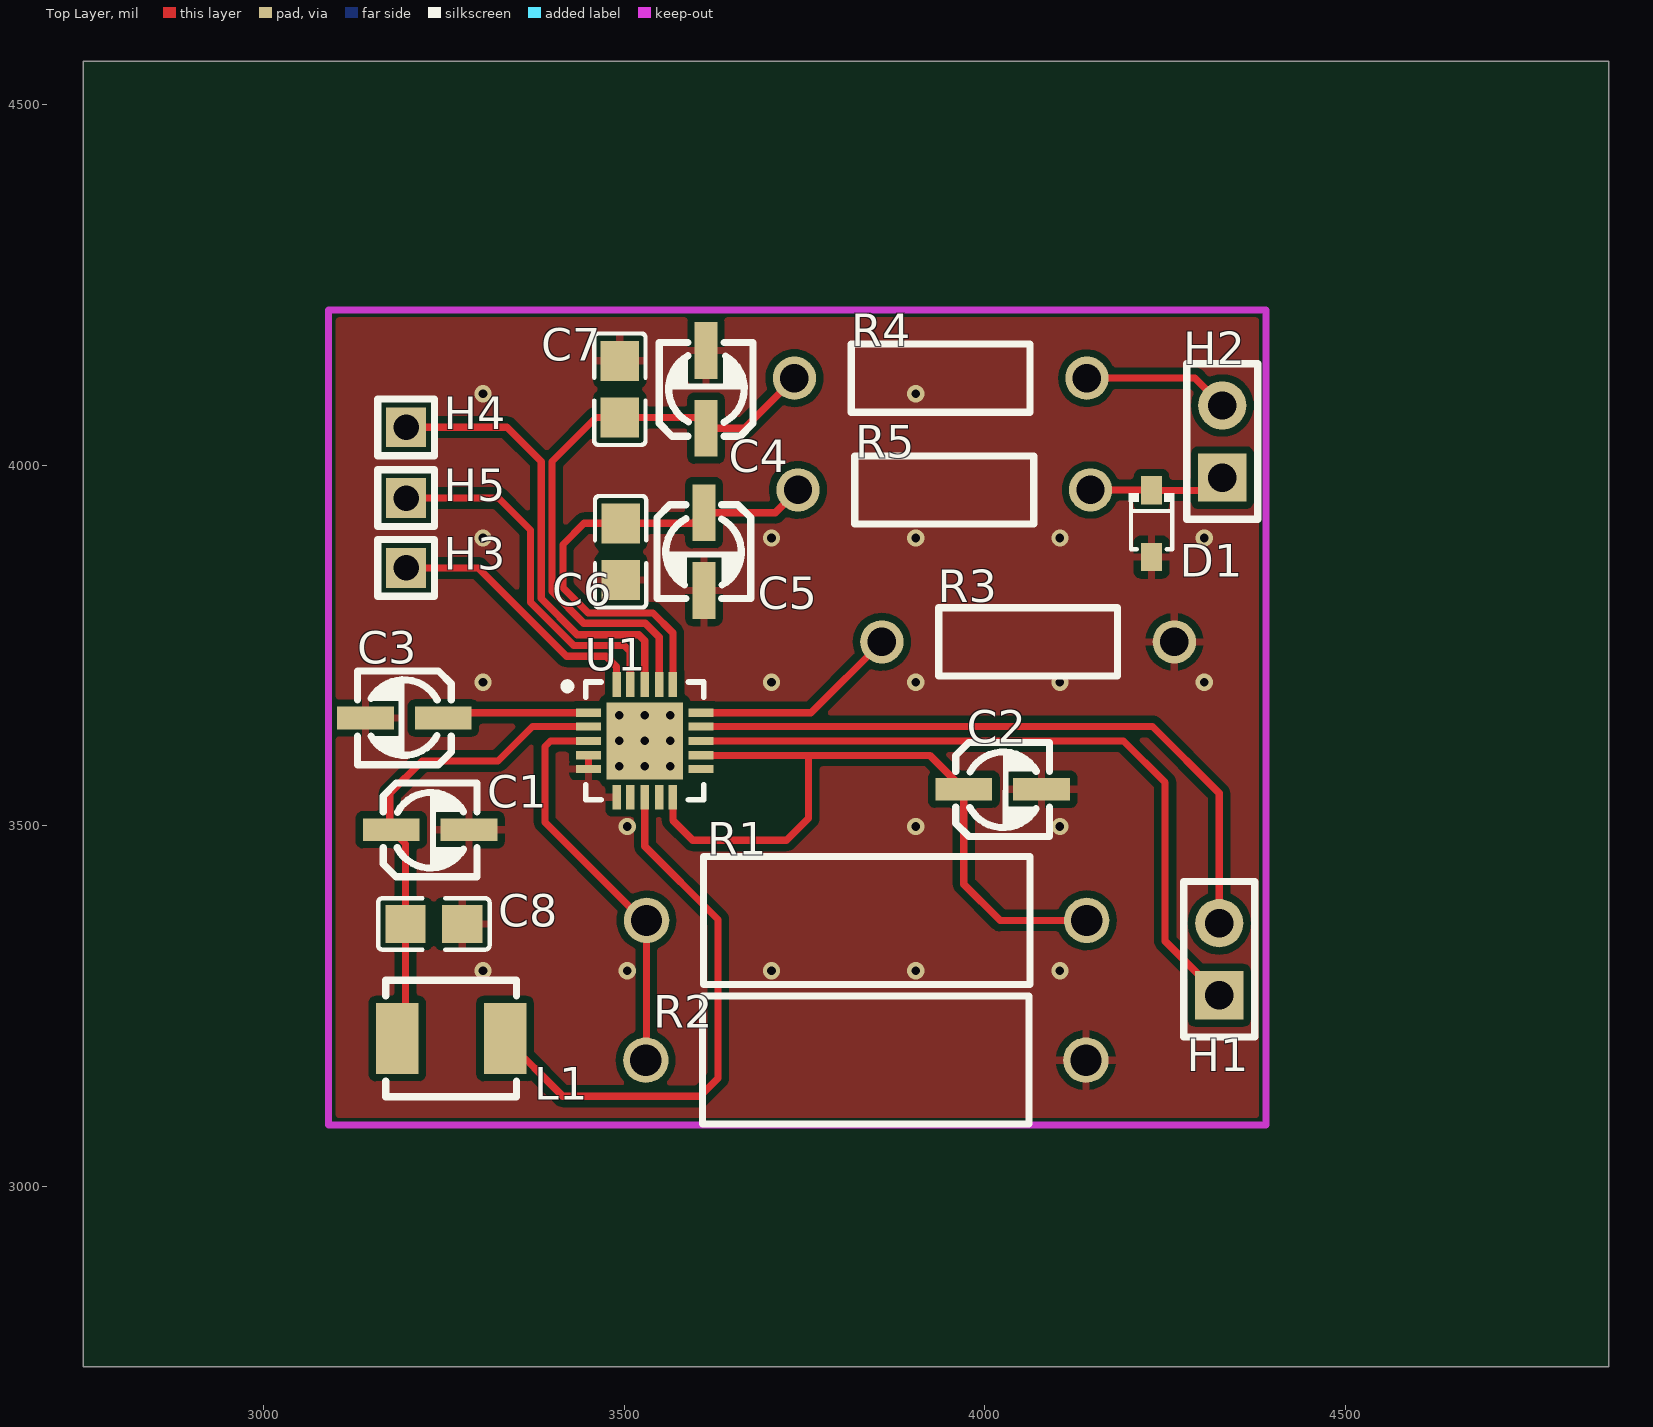
[diagram p0: Top Layer view]
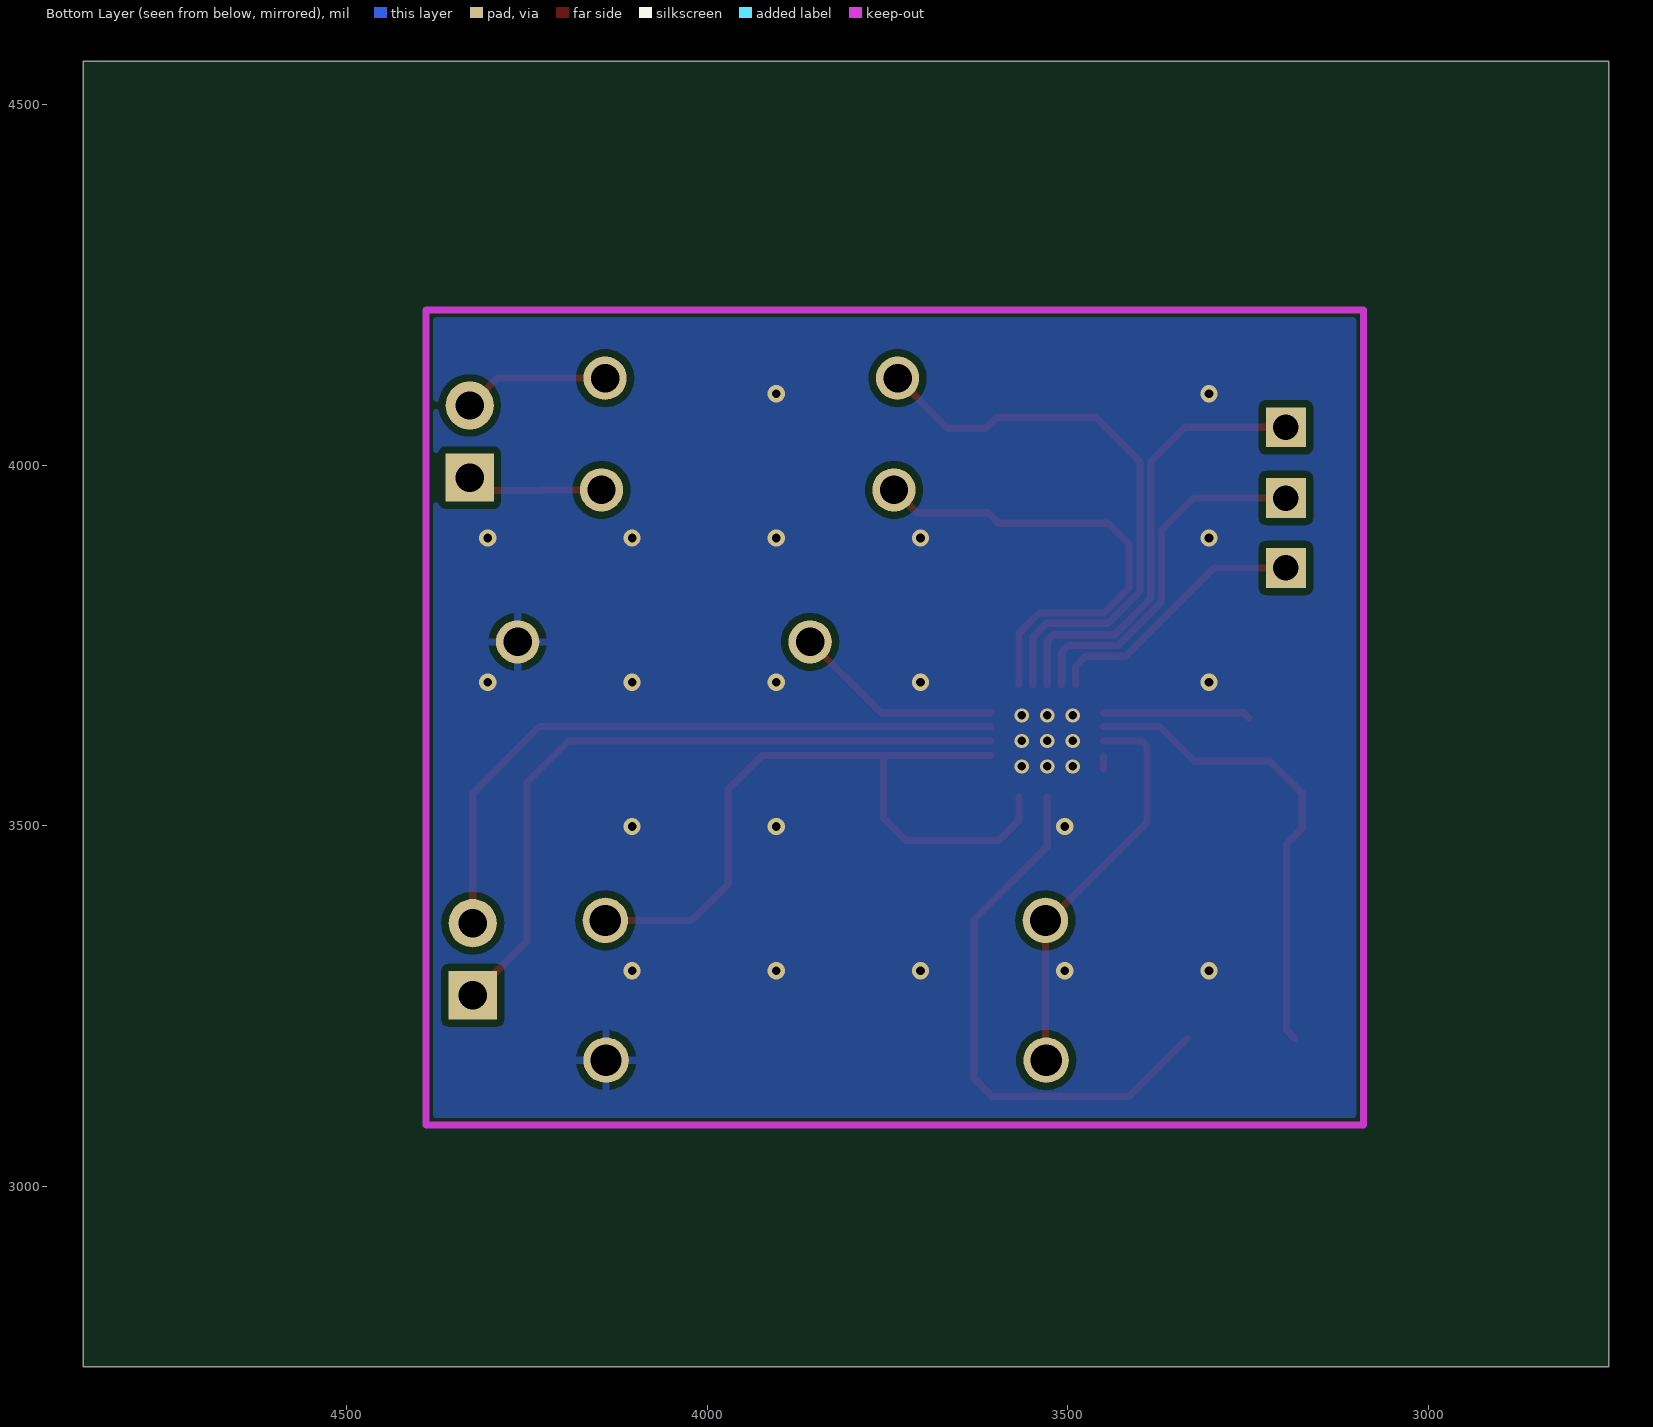
[diagram p1: Bottom Layer view, seen from below]
# Altium PCB MISC51187.pcbdoc
Units mil, origin at the board's own origin, x right, y up, seen from the top; angles counter-clockwise.
Board outline 2115 x 1810 mil, 2 copper layers (Top Layer, Bottom Layer), stack 62.206 mil thick; 21 components, 16 nets, 58 pads, 29 vias.

## Layer stack, top to bottom
Top Solder Mask Layer: solder mask 0.394, Dk 3.3
Top Layer: signal copper 1.379
Dielectric1: surface 59.449, FR4, Dk 4.5
Bottom Layer: signal copper 1.378
Bottom Solder Mask Layer: solder mask 0.394, Dk 3.3

## Board outline
4865,2750 2750,2750 2750,4560 4865,4560

## Design rules (kind name [scope] priority, off if disabled: settings)
BoardOutlineClearance copperThickness2oz_1 [All] p2 off: genericclearance=7.99 ignorepadtopadclearanceinfootprint=FALSE except(0: Arc-SplitContinuation Track-SplitContinuation SMDPad-SplitContinuation THPad-SplitContinuation Via-SplitContinuation Fill-SplitContinuation Region-SplitContinuation Poly-SplitContinuation Text-SplitContinuation Hole-SplitContinuation; 5.98: Arc-CutoutEdge SMDPad-CutoutEdge THPad-CutoutEdge Via-CutoutEdge Fill-CutoutEdge Region-CutoutEdge Text-CutoutEdge; 6.93: Hole-OutlineEdge Hole-CutoutEdge; 10: Poly-OutlineEdge Poly-CutoutEdge; 11.81: Arc-OutlineEdge Track-OutlineEdge SMDPad-OutlineEdge THPad-OutlineEdge Via-OutlineEdge Fill-OutlineEdge Region-OutlineEdge Text-OutlineEdge Track-CutoutEdge)
BoardOutlineClearance copperThickness1oz_1 [All] p4: genericclearance=4.02 ignorepadtopadclearanceinfootprint=FALSE except(0: Arc-SplitContinuation Track-SplitContinuation SMDPad-SplitContinuation THPad-SplitContinuation Via-SplitContinuation Fill-SplitContinuation Region-SplitContinuation Poly-SplitContinuation Text-SplitContinuation Hole-SplitContinuation; 6: SMDPad-CutoutEdge THPad-CutoutEdge Via-CutoutEdge Fill-CutoutEdge Region-CutoutEdge Text-CutoutEdge; 6.93: Hole-OutlineEdge Hole-CutoutEdge; 10: Poly-OutlineEdge Poly-CutoutEdge; 11.8: Arc-OutlineEdge Track-OutlineEdge SMDPad-OutlineEdge THPad-OutlineEdge Via-OutlineEdge Fill-OutlineEdge Region-OutlineEdge Text-OutlineEdge; 11.81: Arc-CutoutEdge Track-CutoutEdge)
Clearance copperThickness2oz [All] p1 off: gap=7.99 ignorepadtopadclearanceinfootprint=FALSE except(5.98: SMDPad-Track SMDPad-SMDPad THPad-Track SMDPad-THPad THPad-THPad Track-Via SMDPad-Via THPad-Via Via-Via Fill-Track Region-Track Fill-SMDPad Region-SMDPad Fill-THPad Region-THPad Fill-Via Region-Via Fill-Fill Fill-Region Region-Region Arc-Track Arc-SMDPad Arc-THPad Arc-Via Fill-Arc Region-Arc Arc-Arc Text-Track SMDPad-Text Text-THPad Text-Via Fill-Text Region-Text Arc-Text Text-Text; 6.93: Hole-Track Hole-SMDPad Hole-THPad Hole-Via Fill-Hole Region-Hole Hole-Arc Hole-Text; 10: Poly-Track Poly-SMDPad Poly-THPad Poly-Via Poly-Fill Poly-Region Poly-Poly Poly-Arc Poly-Text Poly-Hole)
Clearance copperThickness1oz [All] p3: gap=4.02 ignorepadtopadclearanceinfootprint=FALSE except(5.98: SMDPad-Track SMDPad-SMDPad THPad-Track SMDPad-THPad THPad-THPad Track-Via SMDPad-Via THPad-Via Via-Via Fill-Track Region-Track Fill-SMDPad Region-SMDPad Fill-THPad Region-THPad Fill-Via Region-Via Fill-Fill Fill-Region Region-Region; 6: Arc-Track Arc-SMDPad Arc-THPad Arc-Via Fill-Arc Region-Arc Arc-Arc Text-Track SMDPad-Text Text-THPad Text-Via Fill-Text Region-Text Arc-Text Text-Text; 6.93: Hole-Track Hole-SMDPad Hole-THPad Hole-Via Fill-Hole Region-Hole Hole-Arc Hole-Text; 10: Poly-Track Poly-SMDPad Poly-THPad Poly-Via Poly-Fill Poly-Region Poly-Poly Poly-Arc Poly-Text Poly-Hole)
DiffPairsRouting differentialPair [All] p1: maxlimit=6 minlimit=6 mostfreqgap=6 toplayer_minwidth=5 toplayer_prefwidth=10 toplayer_maxwidth=100 toplayer_mingap=6 toplayer_prefgap=6 toplayer_maxgap=6 bottomlayer_minwidth=5 bottomlayer_prefwidth=10 bottomlayer_maxwidth=100 bottomlayer_mingap=6 bottomlayer_prefgap=6 bottomlayer_maxgap=6 maxuncoupledlength=10
HoleToHoleClearance otherClearance [All] p1: gap=11.81 allowstackedmicrovias=TRUE
Length netLength [All] p1: minlimit=0 maxlimit=0
MatchedLengths netLengthTolerance [All] p1: tolerance=1000
PasteMaskExpansion pasteMaskExpansion [All] p1: expansion=0
PlaneConnect innerPlane [All] p1: planeconnectstyle=Relief reliefexpansion=20 reliefentries=4 reliefconductorwidth=10 reliefairgap=10
PolygonConnect copperRegion [(InNet('GND'))] p1: connectstyle=Relief reliefconductorwidth=10 reliefentries=4 polygonreliefangle="90 Angle" airgapwidth=10 via.connectstyle=Relief via.reliefconductorwidth=10 via.reliefentries=4 via.polygonreliefangle="90 Angle" via.airgapwidth=10
RoutingVias viaSize [All] p1: holewidth=12.01 width=24.02 viastyle="Through Hole" minholewidth=11.81 minwidth=19.68 maxholewidth=248.03 maxwidth=393.7
SolderMaskExpansion solderMaskExpansion [IsVia] p1: expansion=-1000 istentingtop=TRUE
SolderMaskExpansion solderMaskExpansion [All] p2: expansion=2 istentingtop=FALSE
Width copperThickness2oz_2 [All] p1 off: maxlimit=100 minlimit=8 preferedwidth=10
Width copperThickness1oz_2 [All] p2: maxlimit=100 minlimit=5 preferedwidth=10

## Components (designator, comment, footprint, x,y, rotation, side; value= is the part's Value field where it differs from the comment)
C1 "0.1uF" C_Ele_SMD_3x5.4mm 3231.07,3493.93 r180 top
C2 "100nF/250V" C_Ele_SMD_3x5.4mm 4025,3550 r180 top
C3 "0.1u" C_Ele_SMD_3x5.4mm 3195,3650 r0 top
C4 "10nF" C_Ele_SMD_3x5.4mm 3613.93,4105.4 r270 top
C5 "10nF" C_Ele_SMD_3x5.4mm 3610,3880 r90 top
C6 "100nF" C0805 3495,3880 r90 top
C7 "100nF" C0805 3493.93,4105.4 r270 top
C8 "10u" C0805 3236.07,3363.93 r180 top
D1 "BAT165E6327" SOD-323_L1.8-W1.3-LS2.5-RD 4231.16,3918.84 r270 top
H1 "" HDR-TH_2P-P2.54-V-F 4325,3315 r90 top
H2 "" HDR-TH_2P-P2.54-V-F 4329.24,4032.82 r90 top
H3 "" HDR-TH_1P-V-M_XKB_X4611WV-01I-C28D40 3197.51,3857.51 r180 top
H4 "" HDR-TH_1P-V-M_XKB_X4611WV-01I-C28D40 3197.51,4052.51 r180 top
H5 "" HDR-TH_1P-V-M_XKB_X4611WV-01I-C28D40 3197.49,3954.45 r180 top
L1 "4.7uH" IND-SMD_L4.6-W4.1-A 3260,3205 r0 top
R1 "1.72M" Res_1W 3836.15,3368.78 r0 top
R2 "15k" Res_1W 3835,3175 r180 top
R3 "18k" Res_1/4W 4060,3755 r180 top
R4 "1k" Res_1/4W 3938.75,4120.69 r180 top
R5 "1k" Res_1/4W 3943.75,3965.69 r180 top
U1 "DRV2700" TI-RGP20-2700X2700TP_V 3528.45,3617.67 r0 top

## Footprints (in the part's own frame and the unit in brackets; to place one, negate y for a bottom-side part, rotate by r counter-clockwise, add the part's x,y. Pads: shape width x height; smd on the part's side, far side on the other; paste and mask are expansions set on the pad)
C0805 [mm]
  rect 1.41x1.35 smd paste-100 mask+0.051: 1(-1,0) 2(1,0)
  silkscreen extent -1.96,-0.9 1.96,0.9
C_Ele_SMD_3x5.4mm [mil]
  rect 78.7x31.5 smd paste+0 mask+2: 1(54.1,-0.55) 2(-53.7,-0.55)
  silkscreen extent -65,-65 65,65
HDR-TH_1P-V-M_XKB_X4611WV-01I-C28D40 [mm]
  rect 1.4x1.4 hole 0.9: 1(0,0)
  silkscreen extent -1,-1 1,1
HDR-TH_2P-P2.54-V-F [mm]
  rect 1.7x1.7 hole 1: 1(-1.27,0)
  round 1.7 hole 1: 2(1.27,0)
  silkscreen extent -2.74,-1.25 2.74,1.25
IND-SMD_L4.6-W4.1-A [mm]
  rect 1.5x2.5 smd: 1(-1.9,0) 2(1.9,0)
  silkscreen extent -2.3,-2.05 2.3,2.05
Res_1/4W [mil]
  round 60 hole 39.37 paste+0 mask+2: 1(-202.76,0) 2(202.76,0)
  silkscreen extent -124,-47 124,47
Res_1W [mm]
  round 1.6 hole 1.1 paste+0 mask+0.051: 1(-7.75,0) 2(7.75,0)
  silkscreen extent -5.75,-2.26 5.75,2.25
SOD-323_L1.8-W1.3-LS2.5-RD [mm]
  rect 1x0.75 smd: 1(-1.173,0) 2(1.173,0)
  silkscreen extent -1.08,-0.8 0.9,0.8
TI-RGP20-2700X2700TP_V [mil]
  rect 34.5x11.5 smd paste+0 mask+4: 1(-78,39) 2(-78,20) 3(-78,0) 4(-78,-20) 5(-78,-39) 11(78,-39) 12(78,-20) 13(78,0) 14(78,20) 15(78,39)
  rect 11.5x34.5 smd paste+0 mask+4: 6(-39,-78) 7(-20,-78) 8(0,-78) 9(20,-78) 10(39,-78) 16(39,78) 17(20,78) 18(0,78) 19(-20,78) 20(-39,78)
  rect 106.5x106.5 smd paste+0 mask+4: 21(0,0)
  silkscreen extent -112,-82 82,82

## Via types
v1: diameter 24.02, hole 12, Top Layer to Bottom Layer, 20 vias
v2: diameter 19.7, hole 11.8, Top Layer to Bottom Layer, 9 vias

## Nets (pads, with @x,y where several pads share a name; then routed paths per layer and width w, separated by ;. In a path a pad name is that pad's centre, name@x,y a point inside that pad or via, vN(x,y) a via of type N, cw(c..) or ccw(c..) an arc to the next point about the centre after c; other vN are vias at no path point)
$1N10: H2.2 R4.1 | length 203.4
  Top Layer w10: R4.1 4291.37,4120.69 H2.2
$1N11: D1.1 H2.1 R5.1 | length 190.4
  Top Layer w10: R5.1 4230.47,3965.69 D1.1 4311.42,3965 H2.1
$1N12: L1.2 U1.8 | length 770.4
  Top Layer w10: L1.2 3414.8,3125 3605,3125 3630,3150 3630,3370 3528.45,3471.55 U1.8
$1N13: H1.2 U1.14 | length 936.9
  Top Layer w10: U1.14 4232.33,3637.67 4325,3545 H1.2
$1N14: H1.1 U1.13 | length 993.5
  Top Layer w10: U1.13 4192.33,3617.67 4250,3560 4250,3340 H1.1
$1N16: R3.2 U1.15 | length 291.5
  Top Layer w10: U1.15 3758.91,3656.67 R3.2
$1N17: R1.1 R2.2 U1.3 | length 560.3
  Top Layer w10: U1.3 3397.67,3617.67 3390,3610 3390,3505 3526.22,3368.78 R1.1 3531.03,3176.15 R2.2
$1N18: C5.1 C6.2 R5.2 U1.16 | length 667.5
  Top Layer w10: U1.16 3567.45,3767.55 3540,3795 3450,3795 3415,3830 3415,3890 3444.37,3919.37 C6.2 3595.82,3919.37 C5.1 3709.4,3934.1 R5.2
$1N19: C4.1 C7.2 R4.2 U1.17 | length 816.7
  Top Layer w10: U1.17 3548.45,3761.55 3529.02,3780.98 3444.02,3780.98 3400,3825 3400,4005 3461.03,4066.03 C7.2 3598.64,4066.03 C4.1 3666.6,4051.3 R4.2
$1N20: H5.1 U1.19 | length 503.6
  Top Layer w10: H5.1 3325.55,3954.45 3370,3910 3370,3810 3430,3750 3500,3750 3508.45,3741.55 U1.19
$1N21: H4.1 U1.18 | length 625.7
  Top Layer w10: H4.1 3337.49,4052.51 3385,4005 3385,3815 3435,3765 3520,3765 3528.45,3756.55 U1.18
$1N22: H3.1 U1.20 | length 373.6
  Top Layer w10: H3.1 3297.49,3857.51 3420,3735 3475,3735 3489.45,3720.55 U1.20
$1N23: C3.1 U1.1 | length 204.3
  Top Layer w10: C3.1 3256.32,3656.67 U1.1
$1N24: C2.1 R1.2 U1.10 U1.12 | length 1038
  Top Layer w10: U1.10 3567.45,3507.55 3595,3480 3725,3480 3755.55,3510.55 3755.55,3597.67 ; U1.12 3755.55,3597.67 ; R1.2 4021.22,3368.78 3970.9,3419.1 C2.1 3923.78,3597.67 3755.55,3597.67
GND: C1.2 C2.2 C3.2 C4.2 C5.2 C6.1 C7.1 C8.1 D1.2 R2.1 R3.1 U1.4 U1.5 U1.6 U1.21 | length 19
  Top Layer w10: U1.5 U1.4
  other v1: 3304.1,3299.1 3504.1,3299.1 3704.1,3299.1 3904.1,3299.1 4104.1,3299.1 3504.1,3499.1 3904.1,3499.1 4104.1,3499.1 3304.1,3699.1 3704.1,3699.1 3904.1,3699.1 4104.1,3699.1 4304.1,3699.1 3304.1,3899.1 3704.1,3899.1 3904.1,3899.1 4104.1,3899.1 4304.1,3899.1 3304.1,4099.1 3904.1,4099.1
  other v2: 3493.05,3582.27 3528.45,3582.27 3563.85,3582.27 3493.05,3617.67 3528.45,3617.67 3563.85,3617.67 3493.05,3653.07 3528.45,3653.07 3563.85,3653.07
VCC: C1.1 C8.2 L1.1 U1.2 | length 667.6
  Top Layer w10: L1.1 3196.7,3216.5 C8.2 3196.7,3474.75 C1.1 3175,3496.45 3175,3545 3220,3590 3325,3590 3372.67,3637.67 U1.2
pads on no net: U1.7 U1.9 U1.11

## Polygon pours and split planes (outlines as drawn)
GND on Top Layer (solid, remove dead copper, pour order 0): 3000,4310 3000,3000 4615,3000 4615,4310
GND on Bottom Layer (solid, remove dead copper, pour order 2): 3030,4275 3030,3005 4490,3005 4490,4275

## Keep-outs
Board Outline Layer:
  lines w10: 3090,3085 3090,4215 4390,4215 4390,3085 3090,3085